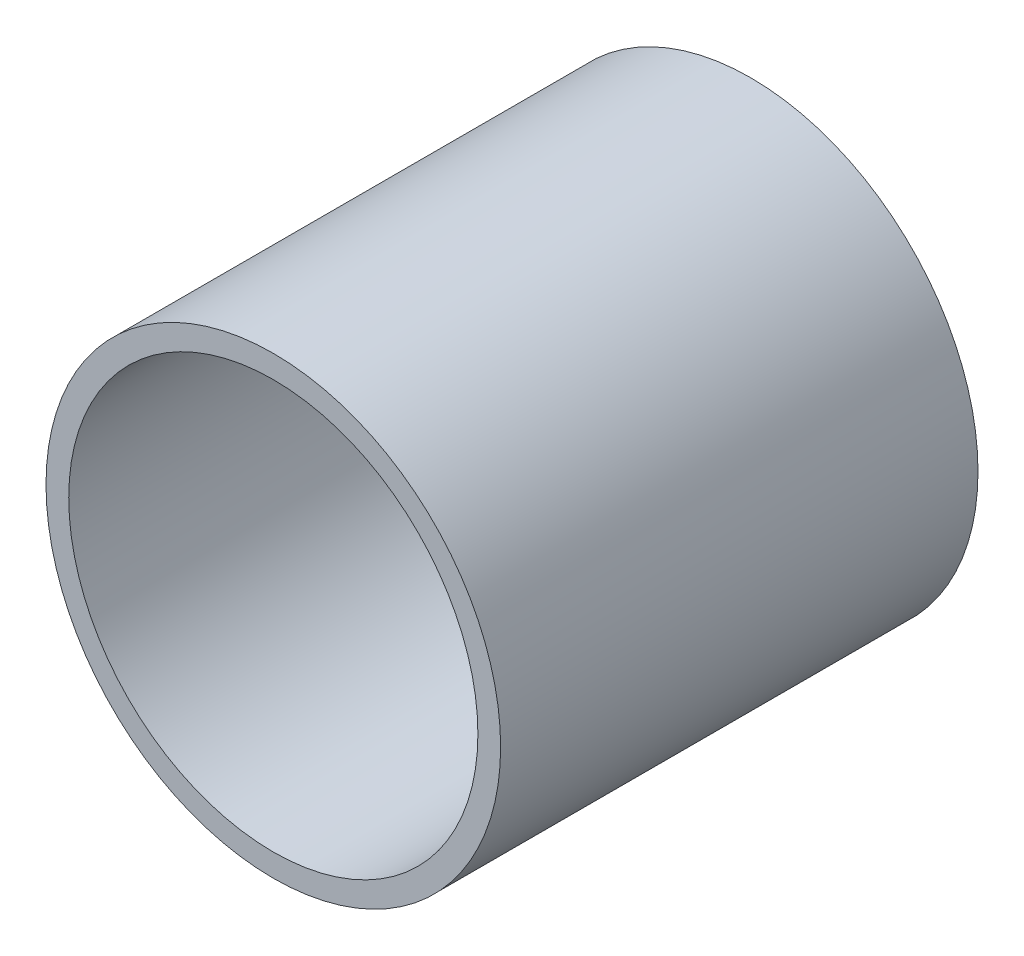
from build123d import *

# Parameters (mm, degrees)
SKETCH1_R           = 10
SKETCH1_R_2         = 9
BOSS_EXTRUDE1_DEPTH = 21


with BuildPart() as part:
    # Sketch1 → Boss-Extrude1 (new body)
    with BuildSketch(Plane.XY):
        with Locations(Location((0, 0, 0), (0, 0, 180))):
            Circle(SKETCH1_R)
        with Locations(Location((0, 0, 0), (0, 0, 180))):
            Circle(SKETCH1_R_2, mode=Mode.SUBTRACT)
    extrude(amount=BOSS_EXTRUDE1_DEPTH)


solid = part.part
